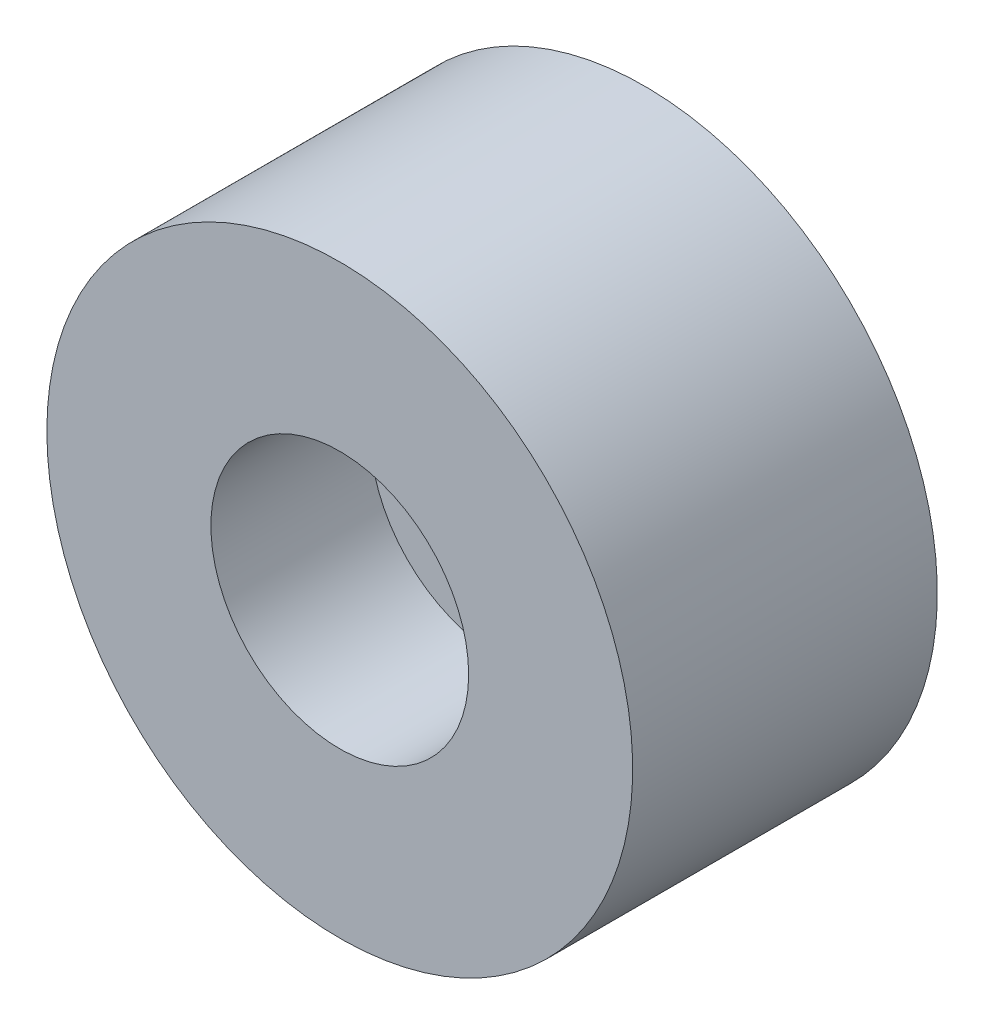
SolidWorks part; units mm, degrees
ref_plane "前视基准面" through (0, 0, 0) normal (0, 0, 1) x (1, 0, 0)
ref_plane "上视基准面" through (0, 0, 0) normal (0, 1, 0) x (1, 0, 0)
ref_plane "右视基准面" through (0, 0, 0) normal (1, 0, 0) x (0, 0, -1)
sketch "草图1" plane through (0, 0, 0) normal (0, 0, 1) x (1, 0, 0)
  circle A0 centre (0, 0) radius 12.5
  dimension "D1" = 25
extrude "凸台-拉伸1" add sketch "草图1" along normal blind 13
sketch "草图4" plane through (0, 0, 13) normal (0, 0, 1) x (1, 0, 0)
  point P0 (0, 0)
hole_wizard "M6 六角圆柱头螺钉的柱形沉头孔1" positions "草图4" profile "草图3" counterbore size "M6" standard "GB" end condition through all
sketch "草图3" plane through (0, 0, 13) normal (1, 0, 0) x (0, -1, 0)
  line L0 (0, 0) -> (0, 13)
  line L1 (0, 13) -> (3.3, 13)
  line L3 (3.3, 13) -> (3.3, 6.8)
  line L4 (3.3, 6.8) -> (5.5, 6.8)
  line L5 (5.5, 6.8) -> (5.5, 0)
  line L7 (5.5, 0) -> (0, 0)
  line L11 (0, -6.35) -> (0, 107.95) construction
  dimension "通孔孔直径" = 6.6
  dimension "通孔孔深度" = 13
  dimension "柱形沉头孔直径" = 11
  dimension "柱形沉头孔深度" = 6.8
